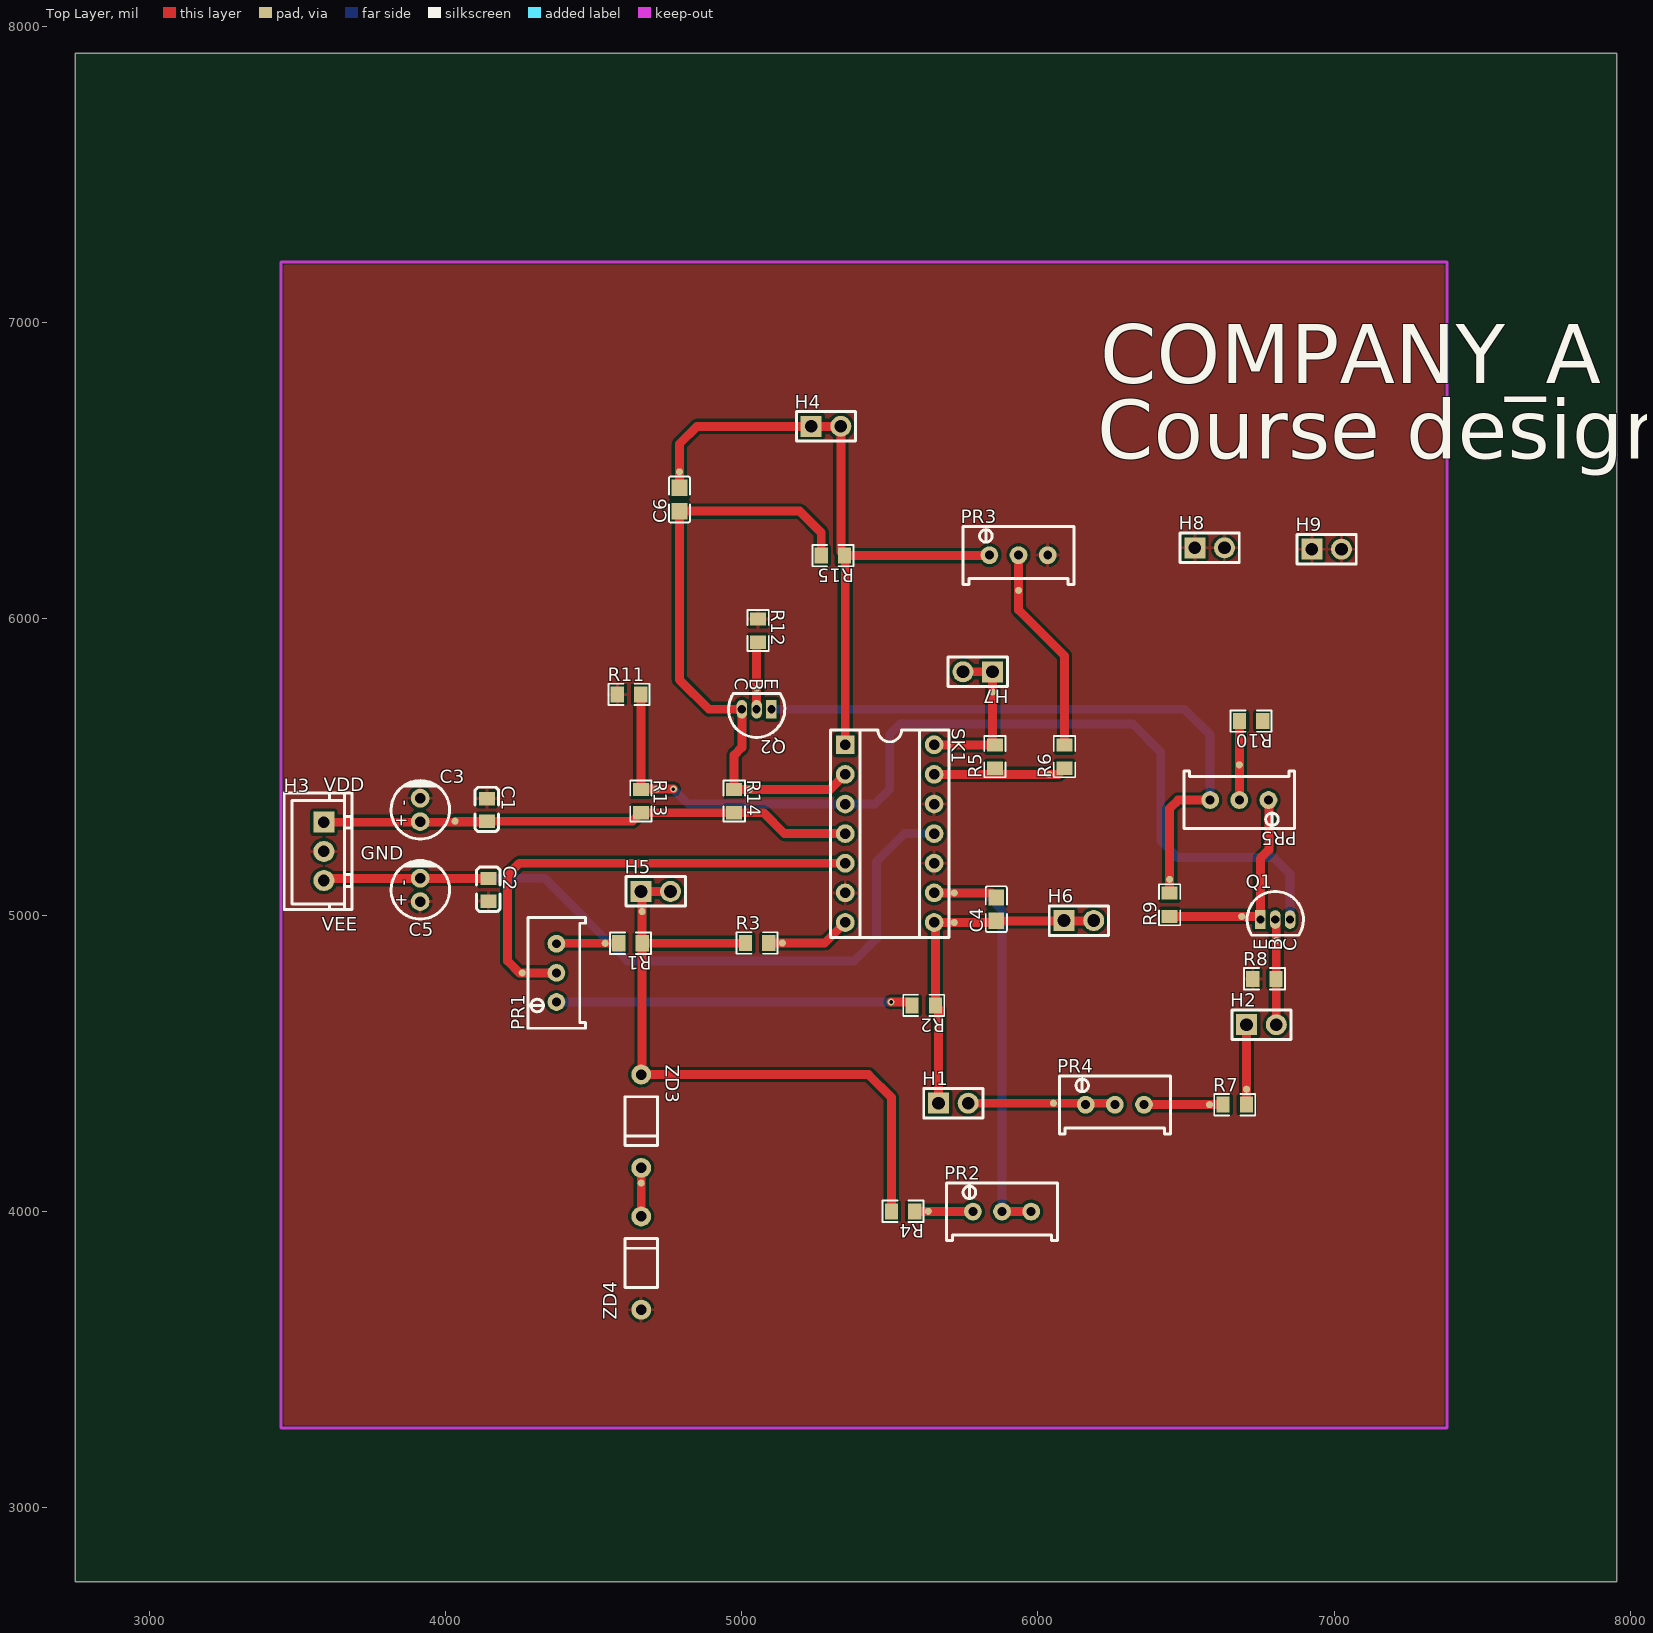
[diagram p0: Top Layer view]
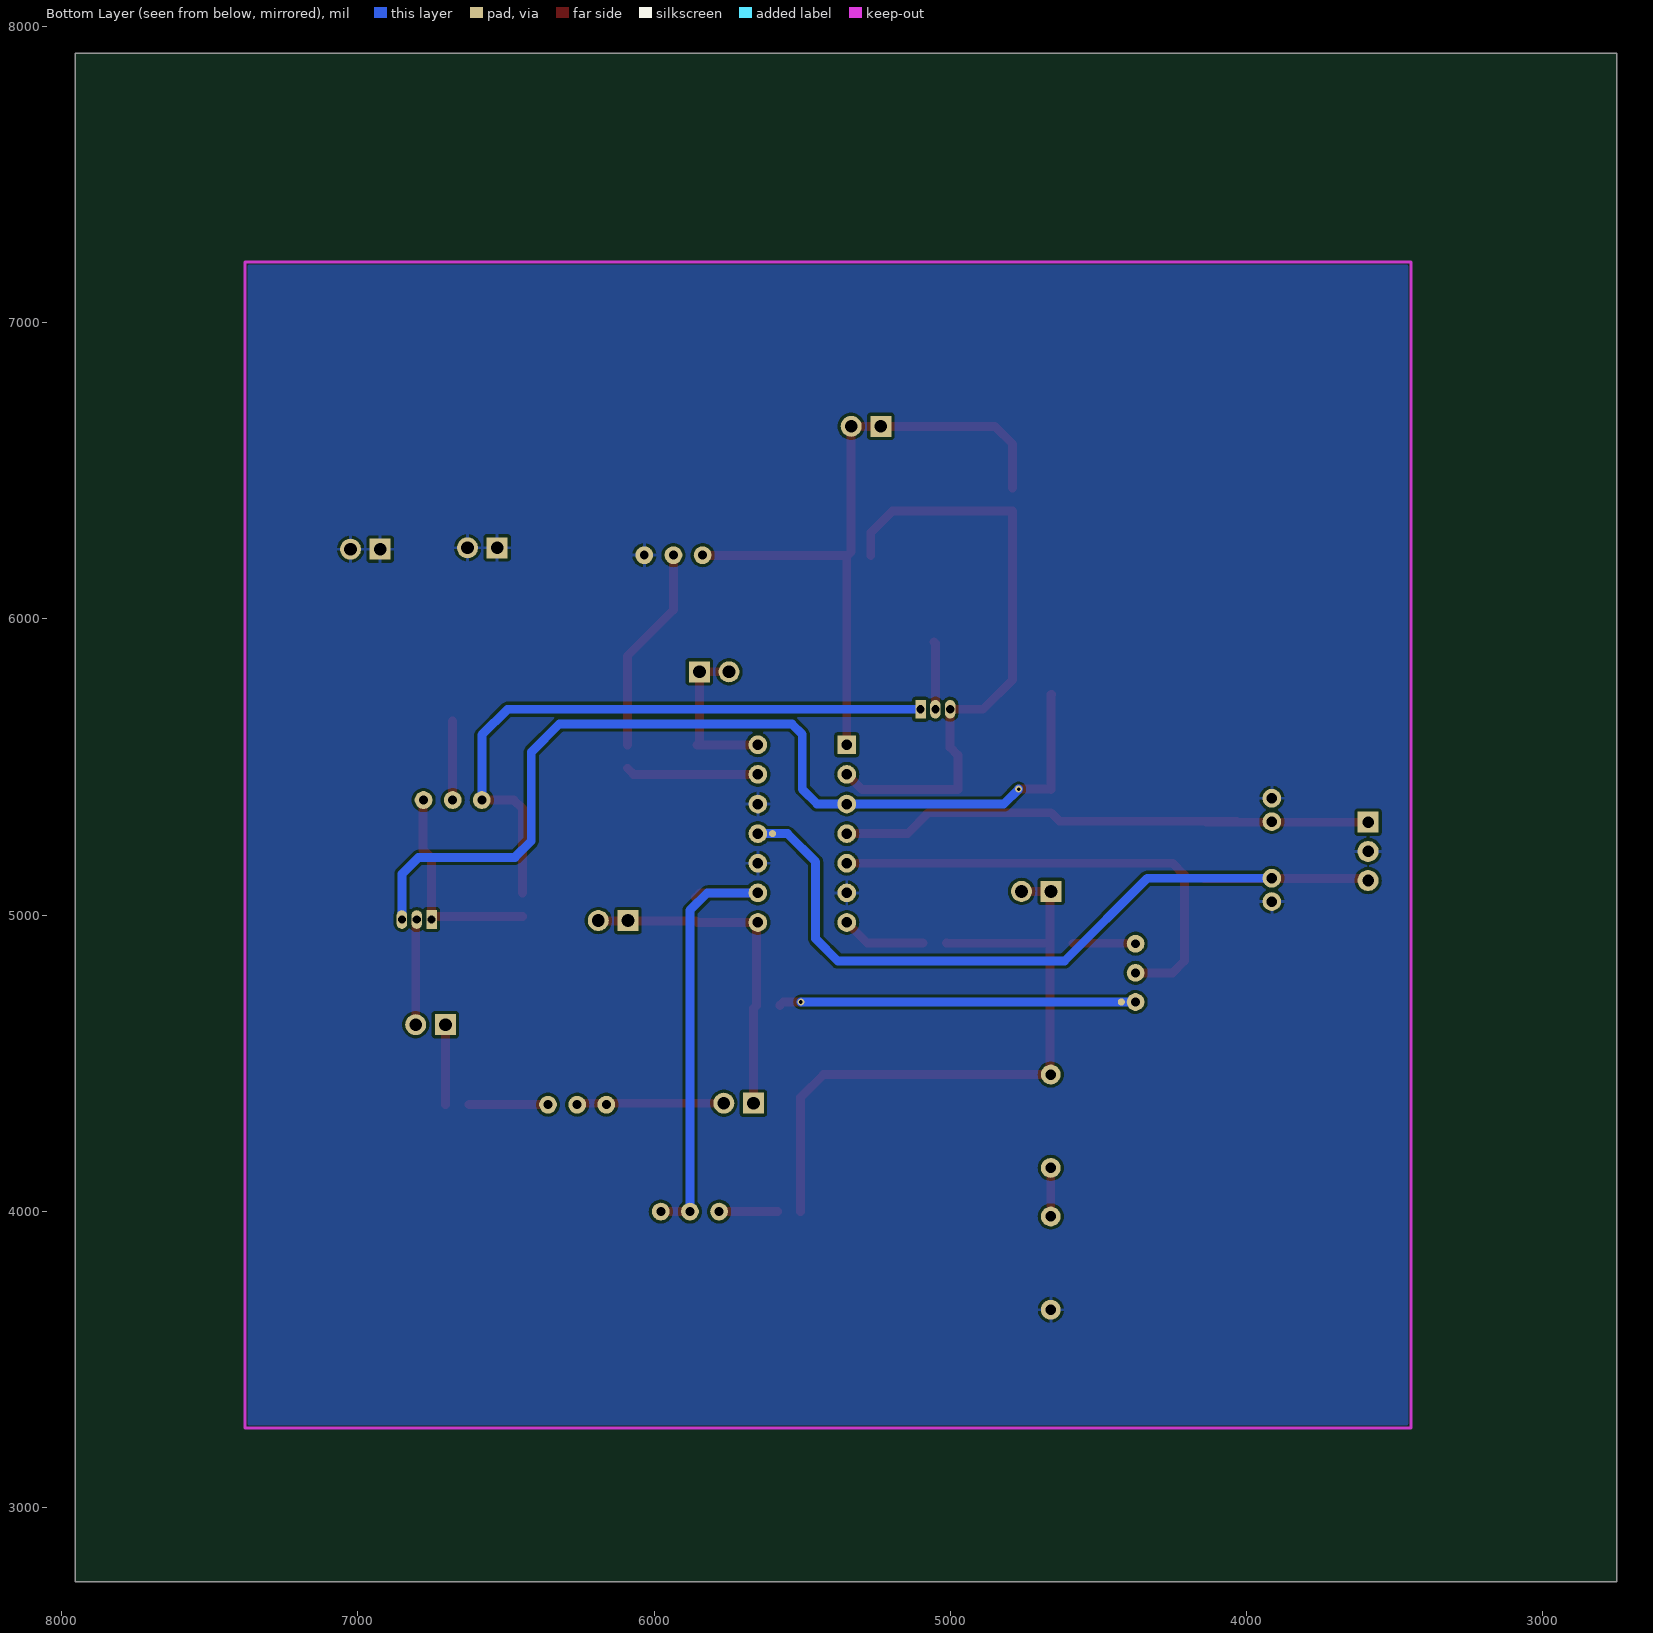
[diagram p1: Bottom Layer view, seen from below]
# Altium PCB MISC51604.pcbdoc
Units mil, origin at the board's own origin, x right, y up, seen from the top; angles counter-clockwise.
Board outline 5205 x 5160 mil, 2 copper layers (Top Layer, Bottom Layer), stack 62.206 mil thick; 40 components, 27 nets, 125 pads, 2 vias.

## Layer stack, top to bottom
Top Solder Mask Layer: solder mask 0.394, Dk 3.3
Top Layer: signal copper 1.379
Dielectric1: surface 59.449, FR4, Dk 4.5
Bottom Layer: signal copper 1.378
Bottom Solder Mask Layer: solder mask 0.394, Dk 3.3

## Board outline
7955,2750 2750,2750 2750,7910 7955,7910

## Design rules (kind name [scope] priority, off if disabled: settings)
BoardOutlineClearance copperThickness2oz_1 [All] p2 off: genericclearance=7.99 ignorepadtopadclearanceinfootprint=FALSE except(0: Arc-SplitContinuation Track-SplitContinuation SMDPad-SplitContinuation THPad-SplitContinuation Via-SplitContinuation Fill-SplitContinuation Region-SplitContinuation Poly-SplitContinuation Text-SplitContinuation Hole-SplitContinuation; 5.98: Arc-CutoutEdge SMDPad-CutoutEdge THPad-CutoutEdge Via-CutoutEdge Fill-CutoutEdge Region-CutoutEdge Text-CutoutEdge; 6.93: Hole-OutlineEdge Hole-CutoutEdge; 10: Poly-OutlineEdge Poly-CutoutEdge; 11.81: Arc-OutlineEdge Track-OutlineEdge SMDPad-OutlineEdge THPad-OutlineEdge Via-OutlineEdge Fill-OutlineEdge Region-OutlineEdge Text-OutlineEdge Track-CutoutEdge)
BoardOutlineClearance copperThickness1oz_1 [All] p4: genericclearance=4.02 ignorepadtopadclearanceinfootprint=FALSE except(0: Arc-SplitContinuation Track-SplitContinuation SMDPad-SplitContinuation THPad-SplitContinuation Via-SplitContinuation Fill-SplitContinuation Region-SplitContinuation Poly-SplitContinuation Text-SplitContinuation Hole-SplitContinuation; 6: SMDPad-CutoutEdge THPad-CutoutEdge Via-CutoutEdge Fill-CutoutEdge Region-CutoutEdge Text-CutoutEdge; 6.93: Hole-OutlineEdge Hole-CutoutEdge; 10: Poly-OutlineEdge Poly-CutoutEdge; 11.8: Arc-OutlineEdge Track-OutlineEdge SMDPad-OutlineEdge THPad-OutlineEdge Via-OutlineEdge Fill-OutlineEdge Region-OutlineEdge Text-OutlineEdge; 11.81: Arc-CutoutEdge Track-CutoutEdge)
Clearance copperThickness2oz [All] p1 off: gap=7.99 ignorepadtopadclearanceinfootprint=FALSE except(5.98: SMDPad-Track SMDPad-SMDPad THPad-Track SMDPad-THPad THPad-THPad Track-Via SMDPad-Via THPad-Via Via-Via Fill-Track Region-Track Fill-SMDPad Region-SMDPad Fill-THPad Region-THPad Fill-Via Region-Via Fill-Fill Fill-Region Region-Region Arc-Track Arc-SMDPad Arc-THPad Arc-Via Fill-Arc Region-Arc Arc-Arc Text-Track SMDPad-Text Text-THPad Text-Via Fill-Text Region-Text Arc-Text Text-Text; 6.93: Hole-Track Hole-SMDPad Hole-THPad Hole-Via Fill-Hole Region-Hole Hole-Arc Hole-Text; 10: Poly-Track Poly-SMDPad Poly-THPad Poly-Via Poly-Fill Poly-Region Poly-Poly Poly-Arc Poly-Text Poly-Hole)
Clearance copperThickness1oz [All] p3: gap=4.02 ignorepadtopadclearanceinfootprint=FALSE except(5.98: SMDPad-Track SMDPad-SMDPad THPad-Track SMDPad-THPad THPad-THPad Track-Via SMDPad-Via THPad-Via Via-Via Fill-Track Region-Track Fill-SMDPad Region-SMDPad Fill-THPad Region-THPad Fill-Via Region-Via Fill-Fill Fill-Region Region-Region; 6: Arc-Track Arc-SMDPad Arc-THPad Arc-Via Fill-Arc Region-Arc Arc-Arc Text-Track SMDPad-Text Text-THPad Text-Via Fill-Text Region-Text Arc-Text Text-Text; 6.93: Hole-Track Hole-SMDPad Hole-THPad Hole-Via Fill-Hole Region-Hole Hole-Arc Hole-Text; 10: Poly-Track Poly-SMDPad Poly-THPad Poly-Via Poly-Fill Poly-Region Poly-Poly Poly-Arc Poly-Text Poly-Hole)
DiffPairsRouting differentialPair [All] p1: maxlimit=6 minlimit=6 mostfreqgap=6 toplayer_minwidth=5 toplayer_prefwidth=10 toplayer_maxwidth=100 toplayer_mingap=6 toplayer_prefgap=6 toplayer_maxgap=6 bottomlayer_minwidth=5 bottomlayer_prefwidth=10 bottomlayer_maxwidth=100 bottomlayer_mingap=6 bottomlayer_prefgap=6 bottomlayer_maxgap=6 maxuncoupledlength=10
HoleToHoleClearance otherClearance [All] p1: gap=11.81 allowstackedmicrovias=TRUE
Length netLength [All] p1: minlimit=0 maxlimit=0
MatchedLengths netLengthTolerance [All] p1: tolerance=1000
PasteMaskExpansion pasteMaskExpansion [All] p1: expansion=0
PlaneConnect innerPlane [All] p1: planeconnectstyle=Relief reliefexpansion=20 reliefentries=4 reliefconductorwidth=10 reliefairgap=10
PolygonConnect copperRegion [(InNet('GND'))] p1: connectstyle=Relief reliefconductorwidth=10 reliefentries=4 polygonreliefangle="90 Angle" airgapwidth=10 via.connectstyle=Relief via.reliefconductorwidth=10 via.reliefentries=4 via.polygonreliefangle="90 Angle" via.airgapwidth=10
RoutingVias viaSize [All] p1: holewidth=12.01 width=24.02 viastyle="Through Hole" minholewidth=11.81 minwidth=19.68 maxholewidth=248.03 maxwidth=393.7
SolderMaskExpansion solderMaskExpansion [IsVia] p1: expansion=-1000 istentingtop=TRUE
SolderMaskExpansion solderMaskExpansion [All] p2: expansion=2 istentingtop=FALSE
Width copperThickness2oz_2 [All] p1 off: maxlimit=100 minlimit=8 preferedwidth=10
Width copperThickness1oz_2 [All] p2: maxlimit=100 minlimit=5 preferedwidth=10

## Components (designator, comment, footprint, x,y, rotation, side; value= is the part's Value field where it differs from the comment)
C1 "100nF" L0805 4140,5355 r270 top
C2 "100nF" L0805 4145,5085 r270 top
C3 "10uF" CAP-TH_BD5.0-P2.00-D0.5-FD-A 3915,5355 r90 top
C4 "22nF" C0805 5860,5020 r90 top
C5 "10uF" CAP-TH_BD5.0-P2.00-D0.5-FD-A 3915,5085 r90 top
C6 "100pF" C0805 4790.2,6402.96 r90 top
H1 "" HDR-TH_2P-P2.54-V-M-1 5715,4365 r0 top
H2 "" HDR-TH_2P-P2.54-V-M-1 6755,4630 r0 top
H3 "" CONN-TH_3P-P2.50_HX-XH2.54-3PZZ-B 3590,5215 r90 top
H4 "" HDR-TH_2P-P2.54-V-M-1 5285,6650 r0 top
H5 "" HDR-TH_2P-P2.54-V-M-1 4710,5080 r0 top
H6 "" HDR-TH_2P-P2.54-V-M-1 6138.6,4981.41 r0 top
H7 "" HDR-TH_2P-P2.54-V-M-1 5797.47,5821.41 r180 top
H8 "" HDR-TH_2P-P2.54-V-M-1 6580,6240 r0 top
H9 "" HDR-TH_2P-P2.54-V-M-1 6975,6235 r0 top
PR1 "5kΩ" R_3296 4370,4805 r90 top
PR2 "100kΩ" R_3296 5879.25,4004.15 r0 top
PR3 "10kΩ" R_3296 5935,6220 r0 top
PR4 "10kΩ" R_3296 6260,4365 r0 top
PR5 "10kΩ" R_3296 6680.21,5383.39 r180 top
Q1 "" S8050_TO_92 6801.51,4984.94 r0 top
Q2 "" S8050_TO_92 5050.87,5694.94 r180 top
R1 "20K" R0805 4625,4905 r180 top
R2 "20K" R0805 5615,4695 r180 top
R3 "1K" R0805 5052.39,4905.75 r0 top
R4 "4.7K" R0805 5545,4000 r180 top
R5 "12K" R0805 5855,5535 r90 top
R6 "10K" R0805 6090,5535 r90 top
R7 "2.2K" R0805 6665,4360 r0 top
R8 "220" R0805 6765,4785 r0 top
R9 "390" R0805 6445,5035 r90 top
R10 "10K" R0805 6720,5655 r180 top
R11 "4.7K" R0805 4620,5745 r0 top
R12 "220" R0805 5055.63,5960.63 r270 top
R13 "4.7K" R0805 4660,5385 r270 top
R14 "4.7K" R0805 4975,5385 r270 top
R15 "4.7K" R0805 5308.31,6213.59 r180 top
SK1 "LM324" DIP-14_L17.8-W10.2-P2.54-BL 5500,5275 r270 top
ZD3 "1N4733A" DO-41_BD2.8-L4.2-P8.00-D0.7-FD 4661.15,4304.15 r270 top
ZD4 "1N4733A" DO-41_BD2.8-L4.2-P8.00-D0.7-FD 4661.15,3825.2 r90 top

## Footprints (in the part's own frame and the unit in brackets; to place one, negate y for a bottom-side part, rotate by r counter-clockwise, add the part's x,y. Pads: shape width x height; smd on the part's side, far side on the other; paste and mask are expansions set on the pad)
C0805 [mm]
  rect 1.41x1.35 smd paste-100 mask+0.051: 1(-1,0) 2(1,0)
  silkscreen extent -1.96,-0.9 1.96,0.9
CAP-TH_BD5.0-P2.00-D0.5-FD-A [mm]
  round 1.6 hole 0.9 paste+0 mask+0.05: 1(-1,0) 2(1,0)
  silkscreen extent -2.49,-2.52 2.6,2.49
CONN-TH_3P-P2.50_HX-XH2.54-3PZZ-B [mm]
  rect 1.8x1.8 hole 1 paste+0 mask+0.05: 1(2.5,0)
  round 1.8 hole 1 paste+0 mask+0.05: 2(0,0) 3(-2.5,0)
  silkscreen extent -5,-2.4 5,3.4
DIP-14_L17.8-W10.2-P2.54-BL [mil]
  rect 63x63 hole 35.43: 1(-300,-150)
  round 63 hole 35.43: 2(-200,-150) 3(-100,-150) 4(0,-150) 5(100,-150) 6(200,-150) 7(300,-150) 8(300,150) 9(200,150) 10(100,150) 11(0,150) 12(-100,150) 13(-200,150) 14(-300,150)
  silkscreen extent -350,-200 350,200
DO-41_BD2.8-L4.2-P8.00-D0.7-FD [mm]
  round 1.7 hole 0.9: 1(-4,0) 2(4,0)
  silkscreen extent -2.1,-1.4 2.1,1.4
HDR-TH_2P-P2.54-V-M-1 [mm]
  rect 1.8x1.8 hole 1.1: 1(-1.27,0)
  round 1.8 hole 1.1: 2(1.27,0)
  silkscreen extent -2.54,-1.27 2.54,1.27
L0805 [mil]
  rect 44.59x54.21 smd paste-3937.01 mask+2: 1(-38.04,0) 2(38.04,0)
  silkscreen extent -77,-40 73,40
R0805 [mm]
  rect 1.133x1.377 smd paste-100 mask+0.051: 1(-1,0) 2(1,0)
  silkscreen extent -1.76,-0.92 1.76,0.92
R_3296 [mil]
  round 60 hole 30 paste+0 mask+2: 1(-98.4,-5) 2(0,-5) 3(98.4,-5)
  silkscreen extent -187,-103 187,92
S8050_TO_92 [mil]
  rect 35.4x63 hole 27.6 paste+0 mask+2: 1(-50,0)
  oval 35.4x63 hole 27.6 paste+0 mask+2: 2(0,0) 3(50,0)
  silkscreen extent -95,-53 95,95

## Free pads (board coordinates)
  round 24 smd: TP1(4033.02,5316.96) TP3(5718,5075) TP4(5718,4975) TP5(4790.2,6496.27) TP6(5027.11,5424.37) TP7(6052.5,4365) TP8(6805,4913.94) TP9(6704.37,4412.11) TP10(4664.37,5012) TP11(5847.47,5753.41) TP12(4259.5,4805) TP14(4539.66,4905) TP15(5630.34,4000) TP16(5935,6096.1) TP17(6579.66,4360) TP18(6680.21,5507.29) TP19(6688.51,4995.63) TP20(6445,5120.34) TP21(4712.11,5425) TP22(5050.87,5765.94) TP23(5137.72,4905.75) TP24(6037.89,5475) TP25(4661.15,4095.22)
  round 24 smd far side: TP2(5600.52,5275) TP13(4422.98,4706.6)

## Via types
v1: diameter 24.02, hole 12, Top Layer to Bottom Layer, 2 vias

## Nets (pads, with @x,y where several pads share a name; then routed paths per layer and width w, separated by ;. In a path a pad name is that pad's centre, name@x,y a point inside that pad or via, vN(x,y) a via of type N, cw(c..) or ccw(c..) an arc to the next point about the centre after c; other vN are vias at no path point)
$1N8: pad.TP12 PR1.2 SK1.5 | length 1628.1
  Top Layer w30: PR1.2 4250,4805 4210,4845 4210,5135 4250,5175 SK1.5
$1N10: pad.TP14 PR1.3 R1.2 | length 211.3
  Top Layer w30: PR1.3 4376.6,4905 pad.TP14 R1.2
$1N12: pad.TP13 PR1.1 R2.2 | length 1205.4
  Top Layer w30: v1(5505,4706.6) 5564.03,4706.6 R2.2
  Bottom Layer w30: PR1.1 v1(5505,4706.6)
$1N18: pad.TP25 ZD3.2 ZD4.2 | length 164
  Top Layer w30: ZD4.2 ZD3.2
$1N21: pad.TP23 R3.2 SK1.7 | length 286.9
  Top Layer w30: R3.2 pad.TP23 5280.75,4905.75 SK1.7
$1N23: pad.TP15 PR2.1 R4.1 | length 196.8
  Top Layer w30: R4.1 pad.TP15 5780,4000 PR2.1
$1N24: C4.2 pad.TP3 PR2.2 PR2.3 SK1.9 | length 1585.3
  Top Layer w30: SK1.9 pad.TP3 5844.37,5075 C4.2 ; PR2.2 PR2.3
  Bottom Layer w30: SK1.9 5820,5075 5879.25,5015.75 PR2.2
$1N27: pad.TP24 R5.1 R6.1 SK1.13 | length 448.5
  Top Layer w30: SK1.13 pad.TP24 6069.37,5475 R6.1
$1N28: pad.TP16 PR3.2 R6.2 | length 704.8
  Top Layer w30: PR3.2 pad.TP16 5935,6030 6090,5875 R6.2
$1N31: H1.2 pad.TP7 PR4.1 PR4.2 | length 497.1
  Top Layer w30: H1.2 pad.TP7 6255,4365 PR4.2
$1N32: pad.TP17 PR4.3 R7.1 | length 267.2
  Top Layer w30: PR4.3 pad.TP17 R7.1
$1N34: H2.1 pad.TP9 R7.2 | length 270.3
  Top Layer w30: R7.2 pad.TP9 6704.37,4629.37 H2.1
$1N36: H2.2 pad.TP8 Q1.2 R8.2 | length 356.4
  Top Layer w30: Q1.2 6805,4981.45 pad.TP8 H2.2
$1N37: pad.TP19 PR5.1 Q1.1 R9.1 | length 726.8
  Top Layer w30: R9.1 pad.TP19 6740.82,4995.63 Q1.1 6751.51,5191.51 6780,5220 6780,5387 PR5.1
$1N38: pad.TP20 PR5.3 Q2.1 R9.2 | length 2170.9
  Top Layer w30: R9.2 pad.TP20 6445,5360 6473.39,5388.39 PR5.3
  Bottom Layer w30: Q2.1 6495.06,5694.94 6581.81,5608.19 PR5.3
$1N39: pad.TP18 PR5.2 R10.2 | length 266.8
  Top Layer w30: PR5.2 pad.TP18 6680.21,5654.58 R10.2
$1N43: pad.TP22 Q2.2 R12.2 | length 228.3
  Top Layer w30: Q2.2 pad.TP22 5050.87,5916.5 R12.2
GND: C1.1 C2.2 C3.2 C5.1 H3.2 H8.1 H8.2 H9.1 H9.2 PR3.3 R8.1 R11.1 R12.1 SK1.6 SK1.10 SK1.12 ZD4.1
NET1: C6.2 H4.1 H4.2 pad.TP5 PR3.1 R15.1 SK1.1 | length 2288.2
  Top Layer w30: C6.2 pad.TP5 4790.2,6590.2 4850,6650 H4.1 H4.2 5335,6226.28 R15.1 ; SK1.1 5350,6211.28 R15.1 ; PR3.1 5835.19,6213.59 R15.1
NET2: C6.1 pad.TP6 Q2.3 R14.1 R15.2 SK1.2 | length 2084.3
  Top Layer w30: R15.2 5268.94,6291.06 5196.41,6363.59 C6.1 4790.2,5794.8 4890.06,5694.94 Q2.3 5000.87,5565.87 4975,5540 R14.1 pad.TP6 5299.37,5424.37 SK1.2
NET3: pad.TP21 Q1.3 R11.2 R13.1 SK1.3 | length 3292.7
  Top Layer w30: R11.2 4660,5744.37 R13.1 4660.63,5425 pad.TP21 v1(4770,5425)
  Bottom Layer w30: v1(4770,5425) 4820,5375 SK1.3 5450,5375 5500,5425 5500,5610 5535,5645 6320,5645 6415,5550 6415,5250 6470,5195 6795,5195 6851.51,5138.49 Q1.3
SIN: H7.1 H7.2 pad.TP11 R5.2 SK1.14 | length 555.4
  Top Layer w30: SK1.14 5650.63,5574.37 R5.2 5847.47,5581.9 pad.TP11 H7.1 H7.2
SOU: H5.1 H5.2 pad.TP10 R1.1 R3.1 R4.2 ZD3.1 | length 2331.3
  Top Layer w30: H5.2 H5.1 4664.37,5075.63 pad.TP10 R1.1 ; R3.1 5012.26,4905 R1.1 ; R4.2 5505.63,4384.37 5428.37,4461.63 ZD3.1 4664.37,4464.84 R1.1
TRI: C4.1 H1.1 H6.1 H6.2 pad.TP4 R2.1 SK1.8 | length 1157.5
  Top Layer w30: H1.1 5665,4684.37 R2.1 5654.37,4970.63 SK1.8 pad.TP4 5854.37,4975 C4.1 6187.82,4980.63 H6.2
VCC: R10.1
VDD: C1.2 C3.1 H3.1 pad.TP1 R13.2 R14.2 SK1.4 | length 1909.6
  Top Layer w30: H3.1 4136.47,5313.43 C1.2 ; pad.TP1 C1.2 ; SK1.4 5145,5275 5074.37,5345.63 R14.2 R13.2 4631.33,5316.96 C1.2
VEE: C2.1 C5.2 H3.3 pad.TP2 SK1.11 | length 2738.8
  Top Layer w30: H3.3 3596.47,5123.04 C2.1
  Bottom Layer w30: C5.2 4335.63,5124.37 4615,4845 5380,4845 5455,4920 5455,5180 5550,5275 SK1.11

## Polygon pours and split planes (outlines as drawn)
GND on Top Layer (solid, remove dead copper, pour order 0): 3000,7660 3000,3000 7705,3000 7705,7660
GND on Bottom Layer (solid, remove dead copper, pour order 2): 3285,7465 3285,3230 7465,3230 7465,7465

## Keep-outs
Board Outline Layer:
  lines w10: 3445,3267.99 3445,7205 7382.01,7205 7382.01,3267.99 3445,3267.99

## Silkscreen, mask and mechanical layers (free items; w line width, h text height)
Top Silkscreen Layer:
  text "COMPANY_A" at 6210,6795 h200
  text "Course design" at 6200,6540 h200
  text "C" at 4977.5,5801.2 h45 r270
  text "B" at 5027.5,5800 h45 r270
  text "E" at 5077.5,5798.7 h45 r270
  text "VDD" at 3589,5417.5 h45
  text "GND" at 3714.55,5187.5 h45
  text "VEE" at 3583.35,4947.5 h45
  text "E" at 6774.88,4881.18 h45 r90
  text "B" at 6824.88,4879.88 h45 r90
  text "C" at 6874.88,4878.68 h45 r90